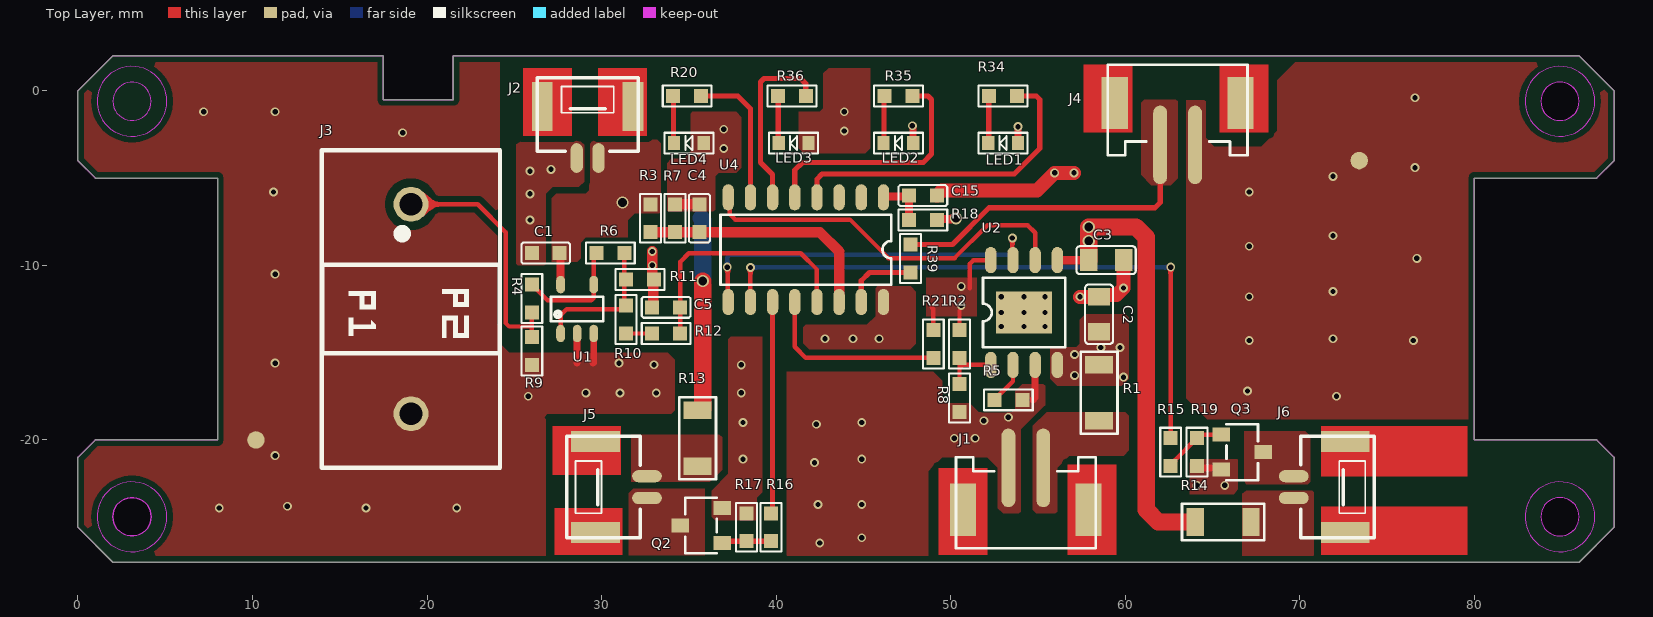
[diagram p0: Top Layer view]
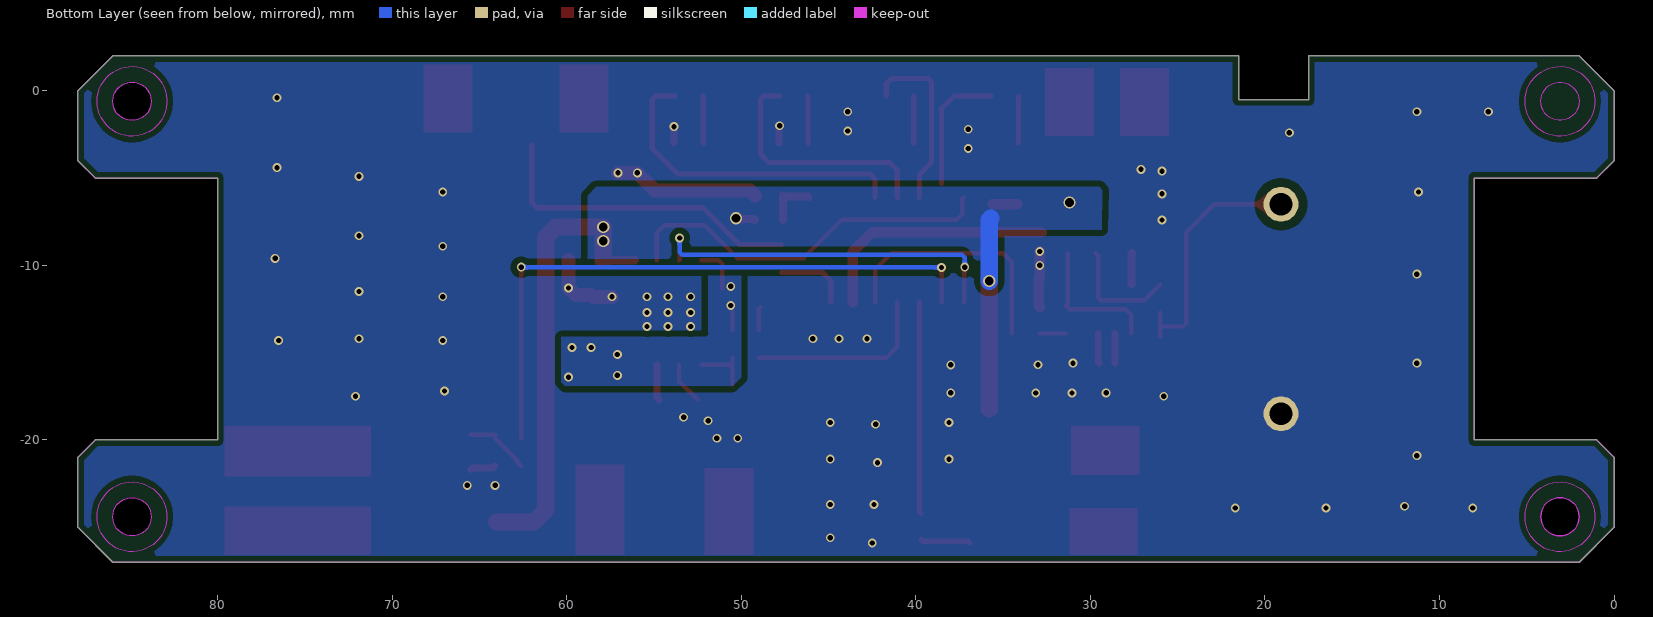
[diagram p1: Bottom Layer view, seen from below]
# Altium PCB MISC84244.PcbDoc
Units mm, origin at the board's own origin, x right, y up, seen from the top; angles counter-clockwise.
Board outline 88 x 29 mm, 2 copper layers (Top Layer, Bottom Layer); 46 components, 36 nets, 130 pads, 93 vias.
Unrouted connection lines stored in the file: 20.

## Layer stack, top to bottom (the 12.6 mil dielectric is the usual default, probably not edited)
Top Solder: solder mask 0.0102, Solder Resist, Dk 3.5
Top Layer: signal copper 0.0356
Dielectric 1: dielectric 0.32, FR-4, Dk 4.8
Bottom Layer: signal copper 0.0356
Bottom Solder: solder mask 0.0102, Solder Resist, Dk 3.5

## Board outline
2,-27 0,-25 0,-21 1,-20 8,-20 8,-5 1,-5 0,-4 0,0 2,2 17.5,2 17.5,-0.5 21.5,-0.5 21.5,2 86,2 88,0 88,-4 87,-5 80,-5 80,-20 87,-20 88,-21 88,-25 86,-27
cut-out: 83.8,-24.4 ccw(c84.9,-24.4) 84.9,-25.5 ccw(c84.9,-24.4) 86,-24.4 ccw(c84.9,-24.4) 84.9,-23.3 ccw(c84.9,-24.4)
cut-out: 83.8,-0.6 ccw(c84.9,-0.6) 84.9,-1.7 ccw(c84.9,-0.6) 86,-0.6 ccw(c84.9,-0.6) 84.9,0.5 ccw(c84.9,-0.6)
cut-out: 3.1,-25.5 cw(c3.1,-24.4) 2,-24.4 cw(c3.1,-24.4) 3.1,-23.3 cw(c3.1,-24.4) 4.2,-24.4 cw(c3.1,-24.4)

## Design rules (kind name [scope] priority, off if disabled: settings)
Clearance [All] p1: gap=0.254 ignorepadtopadclearanceinfootprint=FALSE except(0: Arc-Hole Track-Hole SMDPad-Hole THPad-Hole Via-Hole Fill-Hole Poly-Hole Region-Hole Text-Hole; 0.35: Arc-Fill Arc-Poly Arc-Region Track-Fill Track-Poly Track-Region SMDPad-Fill SMDPad-Poly SMDPad-Region THPad-Fill THPad-Poly THPad-Region Via-Fill Via-Poly Via-Region Fill-Fill Fill-Poly Fill-Region Poly-Poly Poly-Region Region-Region)
PolygonConnect [All] p1: connectstyle=Direct reliefconductorwidth=0.254 reliefentries=4 polygonreliefangle="90 Angle" airgapwidth=0.254
RoutingVias [All] p1: holewidth=0.711 width=1.27 viastyle="Through Hole" minholewidth=0.711 minwidth=1.27 maxholewidth=0.711 maxwidth=1.27
SilkToSilkClearance [All] p1: silktosilkclearance=0
SilkToSolderMaskClearance [IsPad] p1: minsilkscreentomaskgap=0 clearancetoexposedcopper=TRUE
SolderMaskExpansion [All] p1: expansion=0.102 istentingtop=FALSE
SupplyNets "Schematic Supply Nets" [InNet('GND')] p1: voltage=0.000
Width [All] p1: maxlimit=1 minlimit=0.254 preferedwidth=0.254
28 further rules are at their usual default settings.

## Components (designator, comment, footprint, x,y, rotation, side; value= is the part's Value field where it differs from the comment)
C1 "100nF/50V" C0603A 26.8,-9.3 r0 top
C2 "10uF/10V" C0805A 58.5,-12.8 r270 top
C3 "10uF/10V" C0805A 58.9,-9.7 r180 top
C4 "100nF/50V" C0603A 35.6,-7.3 r270 top
C5 "NC" C0603A 33.7,-12.4 r0 top
C15 "1uF/10V" C0603A 48.4,-6 r0 top
J1 "Charge" "HY2.0WT-2A/P 立贴带扣耐温260℃" 54.3,-21.6 r0 top
J2 "Battery" GH1.25-2PIN立贴带扣耐温260℃ 29.2,-3.85 r180 top locked
J3 "Current sensor" IND-TH_L18.2-W10.2-P12.00-D0.9_ZHT103 19.08,-12.5 r270 top locked
J4 "Test port" "HY2.0WT-2A/P 立贴带扣耐温260℃" 63,-3.1 r180 top locked
J5 "Blue LED" GH1.25-2PIN立贴带扣耐温260℃ 32.6,-22.7 r270 top locked
J6 "Yellow LED" GH1.25-2PIN立贴带扣耐温260℃ 69.65,-22.7 r90 top locked
LED1 "25%" LED0603A 53,-3 r0 top locked
LED2 "50%" LED0603A 47,-3 r0 top locked
LED3 "75%" LED0603A 41,-3 r0 top locked
LED4 "100%" LED0603A 35,-3 r0 top locked
Q2 "2N7002" SOT23-3L 35.7,-24.9 r90 top
Q3 "2N7002" SOT23-3L 66.7,-20.7 r270 top
R1 "0.5R/1206" R1206A 58.5,-17.3 r90 top
R2 "NC" R0603A 50.5,-14.5 r90 top
R3 "510K/0603 1%" R0603A 32.8,-7.3 r90 top
R4 "1K/0603" R0603A 26,-11.9 r270 top
R5 "1.2K/0603" R0603A 53.3,-17.7 r180 top
R6 "150K/0603" R0603A 30.5,-9.3 r0 top
R7 "200K/0603 1%" R0603A 34.2,-7.3 r270 top
R8 "NC" R0603A 50.5,-17.6 r90 top
R9 "2K/0603" R0603A 26,-14.9 r270 top
R10 "1K/0603" R0603A 31.4,-13.1 r270 top
R11 "10K/0603" R0603A 32.2,-10.8 r0 top
R12 "0R/0603" R0603A 33.7,-13.9 r0 top
R13 "10R/1206" R1206A 35.5,-19.9 r270 top
R14 "10R/1206" R1206A 65.6,-24.7 r0 top
R15 "1K" R0603A 62.6,-20.7 r90 top
R16 "1K" R0603A 39.7,-25 r90 top
R17 "100K" R0603A 38.3,-25 r270 top
R18 "1R" R0603A 48.4,-7.4 r180 top
R19 "100K" R0603A 64.1,-20.7 r90 top
R20 "100R/5%" R0603A 34.9,-0.3 r0 top
R21 "NC" R0603A 49,-14.5 r90 top
R34 "100R/5%" R0603A 53,-0.3 r0 top
R35 "100R/5%" R0603A 47,-0.3 r0 top
R36 "100R/5%" R0603A 40.9,-0.3 r0 top
R39 "1K" R0603A 47.7,-9.6 r90 top
U1 "LM321" SOT23-5A 28.6,-12.5 r90 top
U2 "4056" ESOP-8L 54.2,-12.7 r90 top
U4 "ZM072" SOP16L 41.7,-9.1 r270 top

## Footprints (in the part's own frame and the unit in brackets; to place one, negate y for a bottom-side part, rotate by r counter-clockwise, add the part's x,y. Pads: shape width x height; smd on the part's side, far side on the other; paste and mask are expansions set on the pad)
C0603A [mm] "贴片电容"
  rect 0.8x0.8 smd mask+0.08: 1(-0.8,0) 2(0.8,0)
  silkscreen extent -1.4,-0.6 1.4,0.6
C0805A [mm] "贴片电容"
  rect 1x1.25 smd: 1(-1,0)
  rect 1x1.25 smd mask+0.102: 2(1,0)
  silkscreen extent -1.7,-0.8 1.7,0.8
ESOP-8L [mm] "贴片MOS/IC"
  rect 2.4x3.2 smd: 0(0,0)
  oval 1.5x0.65 smd: 1(-3,1.905) 2(-3,0.635) 3(-3,-0.635) 4(-3,-1.905) 5(3,-1.905) 6(3,-0.635) 7(3,0.635) 8(3,1.905)
  silkscreen extent -2,-2.35 2,2.35
GH1.25-2PIN立贴带扣耐温260℃ [mm] "立贴带扣耐温260℃"
  rect 1.2x2.8 smd: 0(-2.6,-2.95) 0(2.6,-2.95)
  oval 0.7x1.7 smd: 1(-0.625,0) 2(0.625,0)
  silkscreen extent -2.9,-4.6 2.9,-0.4
"HY2.0WT-2A/P 立贴带扣耐温260℃" [mm] "卧贴连接器"
  rect 1.5x3 smd: 0(-3.6,-2.4) 0(3.6,-2.4)
  oval 0.8x4.5 smd: 1(-1,0) 2(1,0)
  silkscreen extent -4,-4.6 4,0.6
IND-TH_L18.2-W10.2-P12.00-D0.9_ZHT103 [mm]
  round 2 hole 1.3: 1(-6,0) 2(6,0)
  silkscreen extent -9.1,-5.1 9.1,5.1
LED0603A [mm] "贴片LED"
  rect 0.7x0.8 smd: 1(-0.85,0) 2(0.85,0)
  silkscreen extent -1.4,-0.6 1.4,0.6
R0603A [mm] "贴片电阻"
  rect 0.8x0.8 smd mask+0.08: 1(-0.8,0) 2(0.8,0)
  silkscreen extent -1.4,-0.6 1.4,0.6
R1206A [mm] "贴片电阻"
  rect 1x1.6 smd: 1(-1.6,0) 2(1.6,0)
  silkscreen extent -2.35,-1.05 2.35,1.05
SOP16L [mm]
  oval 1.5x0.65 smd: 1(-3,4.445) 2(-3,3.175) 3(-3,1.905) 4(-3,0.635) 5(-3,-0.635) 6(-3,-1.905) 7(-3,-3.175) 8(-3,-4.445) 9(3,-4.445) 10(3,-3.175) 11(3,-1.905) 12(3,-0.635) 13(3,0.635) 14(3,1.905) 15(3,3.175) 16(3,4.445)
  silkscreen extent -2,-4.89 2,4.89
SOT23-3L [mm] "贴片IMOS"
  rect 0.8x1 smd: 1(-1,-1.2) 2(1,-1.2) 3(0,1.2)
  silkscreen extent -1.6,-0.9 1.6,0.9
SOT23-5A [mm] "贴片IC"
  oval 1x0.5 smd mask+0.05: 1(-1.4,0.95) 2(-1.4,0) 3(-1.4,-0.95) 4(1.4,-0.95) 5(1.4,0.95)
  silkscreen extent -0.7,-1.5 0.7,1.5

## Part data
C1 C4 C5: library part Cap0603
C2 C3: library part Cap0805, "SMD capacitor"
C15: library part CH
J1 J2 J3 J4 J5 J6: library part 2PIN, "DC jack right-angle 90° pitch 2.0"
LED1 LED2 LED3 LED4: library part "LED 白发蓝", "SMD LED"
Q2 Q3: "SMD MOSFET"
R1 R13 R14: library part Res1206, "SMD resistor"
R2 R3 R4 R5 R6 R7 R8 R9 R10 R11 R12 R15 R16 R17 R19 R20 R21 R34 R35 R36 R39: library part Res0603, "SMD resistor"
R18: library part RH1
U2: library part TP4056, "Charger IC"
U4: library part MCU-TSSOP-16

## Free pads (board coordinates)
  round 1 smd: 2(10.2,-20) 3(73.4,-4)

## Via types
v1: diameter 0.508, hole 0.305, Top Layer to Bottom Layer, tented both sides, 88 vias
v2: diameter 0.7, hole 0.5, Top Layer to Bottom Layer, tented both sides, 5 vias

## Nets (pads, with @x,y where several pads share a name; then routed paths per layer and width w, separated by ;. In a path a pad name is that pad's centre, name@x,y a point inside that pad or via, vN(x,y) a via of type N, cw(c..) or ccw(c..) an arc to the next point about the centre after c; other vN are vias at no path point)
BAT+: C1.2 C3.2 J2.1 R3.2 R13.1 R14.1 R18.1 U1.5 U2.5 | length 40
  Top Layer w0.45: C1.2 27.64,-9.34 27.64,-11.09 U1.5 ; R18.1 49.252,-7.348 50.252,-7.348 v2(50.3,-7.3)
  Top Layer w0.5: U2.5 C3.2 C3.2@58.1,-9.7
  Top Layer w1: R13.1@35.8,-18.2 v2(35.8,-10.9) ; C3.2 v2(57.9,-8.6) v2(57.9,-7.8) 60.6,-7.8 61.2,-8.4 61.2,-24 61.9,-24.7 R14.1
  Bottom Layer w1: 35.7,-7.3 35.8,-7.4 v2(35.8,-10.9)
  other v2: 31.2,-6.4
CURR: C5.2 R12.2 U4.13 | length 14.4
  Top Layer w0.254: R12.2 C5.2 34.5,-9.8 35,-9.3 41.4,-9.3 42.335,-10.235 U4.13
EN: C2.2 R1.2 R2.2 R21.2 U2.4 U2.8 | length 5.1
  Top Layer w0.254: 48.9,-12.4 49,-12.5 R21.2 ; R2.2 50.5,-12.6 ; 51.1,-11.3 51.1,-9.9 51.3,-9.7 U2.8
  other v1: 59.9,-16.4 57.1,-16.3 57.1,-15.1 58.6,-14.7 59.7,-14.7 50.6,-12.3 50.6,-11.2
FULL: U2.6 U4.8 | length 22.1
  Top Layer w0.254: U4.8 37.331,-6.176 37.331,-7.051 37.655,-7.376 44.226,-7.376 46.432,-9.581 50.219,-9.581 52.1,-7.7 54.4,-7.7 54.835,-8.135 U2.6
GHG: U2.7 U4.9 | length 21.1
  Top Layer w0.254: v1(37.2,-10.1) 37.228,-10.128 37.228,-12.072 U4.9 ; v1(53.532,-8.432) 53.532,-9.667 U2.7
  Bottom Layer w0.254: v1(37.2,-10.1) 37.2,-9.549 37.349,-9.4 53.384,-9.4 53.532,-9.251 v1(53.532,-8.432)
GND: C1.1 C2.1 C3.1 C4.1 C5.1 C15.2 J1.1 J2.2 J3.2 J4.1 LED1.2 LED2.2 LED3.2 LED4.2 pad.2 pad.3 Q2.2 Q3.2 R5.1 R7.1 R8.1 R9.2 R11.2 R17.1 R19.1 U1.2 U1.3 U2.0 U2.3 U4.16 | length 26.3
  Top Layer w0.4: 28.6,-15.6 U1.2 ; 29.5,-15.6 29.55,-15.55 U1.3 ; v1(47.8,-2) 47.8,-2.029 47.85,-2.079 LED2.2 ; LED1.2 v1(53.85,-2.05) ; 54.7,-17.7 54.835,-17.565 U2.3 ; R19.1 64.2,-21.6 65.4,-21.6 Q3.2
  Top Layer w0.6: C5.1 32.95,-12.35 32.95,-10.8 32.9,-10.75 v1(32.9,-9.2) ; R7.1 C4.1
  Top Layer w0.8: C15.2 49.5,-5.7 54.951,-5.7 v1(55.951,-4.7) v1(57.065,-4.7) ; v1(57.4,-11.8) C2.1 58.6,-11.7 59.5,-11.7 v1(59.9,-11.3) C3.1
  other v1: 42.5,-25.9 44.9,-25.6 8.1,-23.9 16.5,-23.9 21.7,-23.9 12,-23.8 42.4,-23.7 44.9,-23.7 64.1,-22.6 65.7,-22.6 42.2,-21.3 38.1,-21.1 44.9,-21.1 11.3,-20.9 50.2,-19.9 51.4,-19.9 42.3,-19.1 38.1,-19 44.9,-19 51.9,-18.9 53.3,-18.7 25.8,-17.5 72.1,-17.5 31.057,-17.315 33.133,-17.315 29.1,-17.3 38,-17.3 67,-17.2 33.006,-15.694 38,-15.7 11.3,-15.6 31,-15.6 67.1,-14.3 76.5,-14.3 42.8,-14.2 44.4,-14.2 45.9,-14.2 71.9,-14.2 52.9,-13.5 54.2,-13.5 55.4,-13.5 52.9,-12.7 54.2,-12.7 55.4,-12.7 52.9,-11.8 54.2,-11.8 55.4,-11.8 67.1,-11.8 71.9,-11.5 11.3,-10.5 32.9,-10 76.7,-9.6 67.1,-8.9 71.9,-8.3 25.9,-7.4 25.9,-5.9 11.2,-5.8 67.1,-5.8 71.9,-4.9 25.9,-4.6 27.1,-4.5 76.6,-4.4 37,-3.3 18.6,-2.4 43.9,-2.3 37,-2.2 7.2,-1.2 11.3,-1.2 43.9,-1.2 76.6,-0.4
ICPCL: U4.3
ICPDA: U4.2
LED1: LED1.1 R34.1 | length 2.7
  Top Layer w0.3: LED1.1 52.175,-2.975 52.175,-0.325 R34.1
LED2: LED2.1 R35.1 | length 2.7
  Top Layer w0.3: LED2.1 46.175,-2.975 46.175,-0.325 R35.1
LED3: LED3.1 R36.1 | length 2.7
  Top Layer w0.3: R36.1 40.125,-0.325 40.125,-2.975 LED3.1
LEDB: R16.2 U4.11 | length 12.1
  Top Layer w0.3: R16.2 39.795,-24.105 U4.11
LEDY: R15.2 U4.10 | length 35.9
  Top Layer w0.254: U4.10 v1(38.525,-10.125) ; R15.2 v1(62.6,-10.1)
  Bottom Layer w0.254: v1(38.525,-10.125) 38.538,-10.112 62.587,-10.112 v1(62.6,-10.1)
NetC15_1: C15.1 R18.2 U4.1 | length 2.9
  Top Layer w0.45: U4.1 46.195,-6.05 47.55,-6.05 C15.1 R18.2
NetJ1_2: J1.2 R1.1
NetJ3_1: J3.1 R4.2 R9.1 | length 14.3
  Top Layer w0.254: J3.1 22.9,-6.5 24.5,-8.1 24.5,-13.3 24.7,-13.5 26,-13.5 ; R9.1 26,-13.5 ; R4.2 26,-13.5
NetJ4_2: J4.2 R39.2 | length 18.6
  Top Layer w0.3: R39.2 50.1,-8.8 52.2,-6.7 61.7,-6.7 62,-6.4 J4.2
NetJ5_1: J5.1 R13.2
NetJ5_2: J5.2 Q2.3
NetJ6_1: J6.1 R14.2
NetJ6_2: J6.2 Q3.3
NetLED4_1: LED4.1 R20.1 | length 2.7
  Top Layer w0.3: R20.1 34.125,-0.325 34.125,-2.975 LED4.1
NetQ2_1: Q2.1 R16.1 R17.2 | length 2.9
  Top Layer w0.3: Q2.1 37,-25.8 R17.2 39.6,-25.8 R16.1@39.7,-25.7
NetQ3_1: Q3.1 R15.1 R19.2 | length 3.6
  Top Layer w0.254: R15.1 62.873,-21.227 62.873,-21.127 R19.2 ; R19.2@64.1,-19.7 Q3.1
NetR2_1: R2.1 R8.2 U2.1 | length 3.4
  Top Layer w0.254: R8.2 50.5,-15.9 ; R2.1 50.5,-15.9 ; U2.1 50.7,-15.7 50.5,-15.9
NetR4_1: R4.1 R6.1 U1.4 | length 6.6
  Top Layer w0.254: R4.1 26.9,-12 29.401,-12 29.55,-11.851 29.55,-9.45 R6.1
NetR5_2: R5.2 U2.2 | length 2.4
  Top Layer w0.254: R5.2 53.565,-16.635 U2.2
NetR6_2: R6.2 R10.1 R11.1 U1.1 | length 8.1
  Top Layer w0.254: U1.1 27.65,-12.85 27.992,-12.508 31.192,-12.508 R10.1 31.3,-12.2 R6.2
NetR10_2: R10.2 R12.1 | length 1.5
  Top Layer w0.254: R10.2 R12.1
NetR20_2: R20.2 U4.7 | length 7.4
  Top Layer w0.3: R20.2 37.8,-0.3 38.525,-1.025 38.525,-5.3
NetR21_1: R21.1 U4.12 | length 10.8
  Top Layer w0.254: U4.12 41.065,-14.665 41.7,-15.3 R21.1
NetR34_2: R34.2 U4.4 | length 18.7
  Top Layer w0.3: U4.4 42.335,-5.065 42.635,-4.765 53.635,-4.765 55.1,-3.3 55.1,-0.5 54.9,-0.3 R34.2
NetR35_2: R35.2 U4.5 | length 14.1
  Top Layer w0.3: U4.5 41.065,-4.535 41.5,-4.1 48.424,-4.1 48.9,-3.624 48.9,-0.5 48.7,-0.3 R35.2
NetR36_2: R36.2 U4.6 | length 10.4
  Top Layer w0.3: U4.6 39.795,-4.795 39.1,-4.1 39.1,0.5 39.3,0.7 41.4,0.7 41.7,0.4 R36.2
NetR39_1: R39.1 U4.15 | length 4.2
  Top Layer w0.3: U4.15 44.875,-10.876 45.351,-10.4 R39.1
VBAT1: C4.2 R3.1 R7.2 U4.14 | length 14.2
  Top Layer w0.6: R3.1 R7.2 C4.2 42.5,-8.1 43.605,-9.205 U4.14
pads on no net: J1.0 J2.0 J4.0 J5.0 J6.0

## Polygon pours and split planes (outlines as drawn)
GND on Top Layer "NONET_L02_P-001" (solid, remove dead copper, pour order 18): 63.5,-0.529 64.529,-0.529 64.6,-0.6 64.6,-2.7 65.1,-3.2 67.8,-3.2 68.7,-2.3 68.7,0.6 70.1,2 88.3,2 88.5,1.8 88.5,-18.3 88,-18.8 64.7,-18.8 63.5,-17.6
GND on Top Layer "NONET_L02_P-001" (solid, remove dead copper, pour order 0): 26.9,-18.5 26.7,-18.7 26.8,-18.8 26.8,-26.8 26,-27.6 2,-27.6 -1.3,-24.3 -1.3,3.9 23.1,3.6 24.16,2.54 24.16,-14.46 24.7,-15 33.8,-15 34.2,-15.4 34.2,-18.3 34,-18.5
NetJ4_2 on Top Layer "NONET_L02_P-001" (solid, remove dead copper, pour order 23): 61.071,-0.5 60.9,-0.671 60.9,-4.8 61.5,-5.4 62.6,-5.4 63,-5 63,-0.6 62.9,-0.5
GND on Top Layer "NONET_L02_P-001" (solid, remove dead copper, pour order 20): 66.443,-21.143 66.443,-22.857 66.2,-23.1 63.7,-23.1 63.7,-21.3 63.9,-21.1 66.4,-21.1
GND on Top Layer "NONET_L02_P-001" (solid, remove dead copper, pour order 19): 45.7,-11.3 45.7,-12.9 45.2,-13.4 43.65,-13.4 41.7,-13.4 41.5,-13.6 41.5,-14.5 41.9,-14.9 47.6,-14.9 48,-14.5 48,-11.5 47.7,-11.2 45.8,-11.2
GND on Top Layer "NONET_L02_P-001" (solid, remove dead copper, pour order 16): 41.3,-1.2 41.3,-3.3 41.6,-3.6 45.1,-3.6 45.4,-3.3 45.4,1.3 43,1.3 42.7,1 42.7,-1 42.5,-1.2 41.4,-1.2
EN on Top Layer "NONET_L02_P-001" (solid, remove dead copper, pour order 14): 48.6,-10.7 48.6,-12.9 51.5,-12.9 51.5,-10.7
GND on Top Layer "NONET_L02_P-001" (solid, remove dead copper, pour order 12): 49,-16.1 49.5,-16.6 49.5,-17.6 49.8,-17.9 51.1,-17.9 51.6,-18.4 53.5,-18.4 53.7,-18.2 53.7,-17.2 54.1,-16.8 55.3,-16.8 55.4,-16.9 55.4,-18 54,-19.4 54,-21.4 54,-22.5 54,-24.1 53.9,-24.2 53,-24.2 52.7,-23.9 52.7,-21.6 52.1,-21 49.5,-21 48.7,-21.8 48.7,-27 41,-27 40.6,-26.6 40.6,-16.1
NetJ1_2 on Top Layer "NONET_L02_P-001" (solid, remove dead copper, pour order 11): 60,-18.4 60.2,-18.6 60.2,-19.4 60.2,-20.6 59.9,-20.9 56.8,-20.9 56.1,-21.6 56.1,-24.1 56,-24.2 54.9,-24.2 54.7,-24 54.7,-19.2 55.5,-18.4
EN on Top Layer "NONET_L02_P-001" (solid, remove dead copper, pour order 10): 55.7,-14.7 55.7,-16.5 56.1,-16.9 59.8,-16.9 60.2,-16.5 60.2,-13 60,-12.8 57.7,-12.8 57.4,-13.1 57.4,-14.5 57.2,-14.7
NetJ6_2 on Top Layer "NONET_L02_P-001" (solid, remove dead copper, pour order 9): 66.8,-19.5 70.3,-19.5 70.6,-19.8 70.6,-22.4 70.4,-22.6 66.8,-22.6
NetJ6_1 on Top Layer "NONET_L02_P-001" (solid, remove dead copper, pour order 8): 70.8,-26.6 70.8,-23 70.7,-22.9 66.933,-22.9 66.7,-23.075 66.7,-26.7 66.9,-26.9 70.5,-26.9
GND on Top Layer "NONET_L02_P-001" (solid, remove dead copper, pour order 6): 35.1,-3.5 34.7,-3.9 34,-3.9 33.7,-4.2 33.7,-6.8 33.812,-6.912 36.388,-6.912 36.5,-6.8 36.5,-4.9 36.7,-4.7 37.7,-4.7 38,-4.4 38,-1.5 37.7,-1.2 35.2,-1.2 35.1,-1.3
GND on Top Layer "NONET_L02_P-001" (solid, remove dead copper, pour order 5): 39.2,-23 38.9,-23.3 38.9,-24.6 36.5,-24.6 36.3,-24.4 36.3,-22.9 37.257,-21.943 37.257,-14.243 37.4,-14.1 39.2,-14.1
NetJ5_1 on Top Layer "NONET_L02_P-001" (solid, remove dead copper, pour order 4): 31.7,-22.4 36.2,-22.4 36.5,-22.1 36.9,-21.7 36.9,-19.85 36.75,-19.7 31.7,-19.7
NetJ5_2 on Top Layer "NONET_L02_P-001" (solid, remove dead copper, pour order 3): 31.55,-26.6 31.55,-23.05 31.8,-22.8 35.9,-22.8 35.9,-26.6
BAT+ on Top Layer "NONET_L02_P-001" (solid, remove dead copper, pour order 2): 27.1,-9.8 28.6,-9.8 28.8,-9.6 28.8,-8.7 29.1,-8.4 31.5,-8.4 31.5,-7.4 31.9,-7 33.3,-7 33.4,-6.9 33.4,-3 33.2,-2.8 29.4,-2.8 29.3,-2.9 29.3,-5.7 29.1,-5.9 27.4,-5.9 27.1,-6.2
GND on Top Layer "NONET_L02_P-001" (solid, remove dead copper, pour order 1): 28.25,-5.5 28.7,-5.5 29,-5.2 29,-3.1 28.7,-2.8 25.2,-2.8 25.1,-2.9 25.1,-9.9 25.2,-10 26.7,-10 26.8,-9.9 26.8,-5.9 27.2,-5.5
GND on Bottom Layer "GND_L02_P015" (solid, remove dead copper, pour order 15): 2,-27 0,-25 0,-21 1,-20 8,-20 8,-5 1,-5 0,-4 0,0 2,2 17.5,2 17.5,-0.5 21.5,-0.5 21.5,2 86,2 88,0 88,-4 87,-5 80,-5 80,-20 87,-20 88,-21 88,-25 86,-27
EN on Bottom Layer "NONET_L02_P-001" (solid, remove dead copper, pour order 13): 50.5,-16.9 50,-16.4 50,-12.9 50,-10.6 50.1,-10.5 51.9,-10.5 51.9,-13.9 51.85,-13.95 52,-14.1 60.3,-14.1 60.3,-16.7 60.1,-16.9
BAT+ on Bottom Layer "NONET_L02_P-001" (solid, remove dead copper, pour order 7): 35.3,-8 35.25,-7.95 29.359,-7.95 29.309,-5.5 58.3,-5.5 58.8,-6 58.8,-9.7 35.7,-9.7 35.3,-9.3

## Keep-outs
Keep-Out Layer:
  circle w0.01: c84.9,-0.6 r2
  circle w0.01: c84.9,-24.4 r2
  circle w0.01: c3.1,-0.6 r2
  circle w0.01: c3.1,-24.4 r2
  circle w0.013: c3.1,-0.6 r1.1
  circle w0.013: c3.1,-24.4 r1.1
  circle w0.013: c84.9,-24.4 r1.1
  circle w0.013: c84.9,-0.6 r1.1
  lines w0.013: 0,-25 2,-27 86,-27 88,-25 88,-21 87,-20 80,-20 80,-5 87,-5 88,-4 88,0 86,2 21.5,2 21.5,-0.5 17.5,-0.5 17.5,2 2,2 0,0 0,-4 1,-5 8,-5 8,-20 1,-20 0,-21 0,-25

## Other copper
Top Layer:
  region: 65.4,1.5 65.4,-2.4 68.2,-2.4 68.2,1.5
  region: 57.6,1.5 57.6,-2.4 60.4,-2.4 60.4,1.5
  region: 25.5,1.3 25.5,-2.6 28.3,-2.6 28.3,1.3
  region: 29.8,1.3 29.8,-2.6 32.6,-2.6 32.6,1.3
  region: 31.1,-19.2 27.2,-19.2 27.2,-22 31.1,-22
  region: 31.2,-23.9 27.3,-23.9 27.3,-26.6 31.2,-26.6
  region: 52.1,-26.6 52.1,-21.6 49.3,-21.6 49.3,-26.6
  region: 59.5,-26.6 59.5,-21.4 56.7,-21.4 56.7,-26.6
  rectangle net GND: 71.2,-22.1 79.6,-19.2
  rectangle: 71.2,-26.6 79.6,-23.8
  pour cut-out: 19.08,-8 cw(c19.08,-6.5) 17.58,-6.5 cw(c19.08,-6.5) 19.08,-5 cw(c19.08,-6.5) 20.58,-6.5 cw(c19.08,-6.5)
Bottom Layer:
  pour cut-out: 19.08,-8 cw(c19.08,-6.5) 17.58,-6.5 cw(c19.08,-6.5) 19.08,-5 cw(c19.08,-6.5) 20.58,-6.5 cw(c19.08,-6.5)